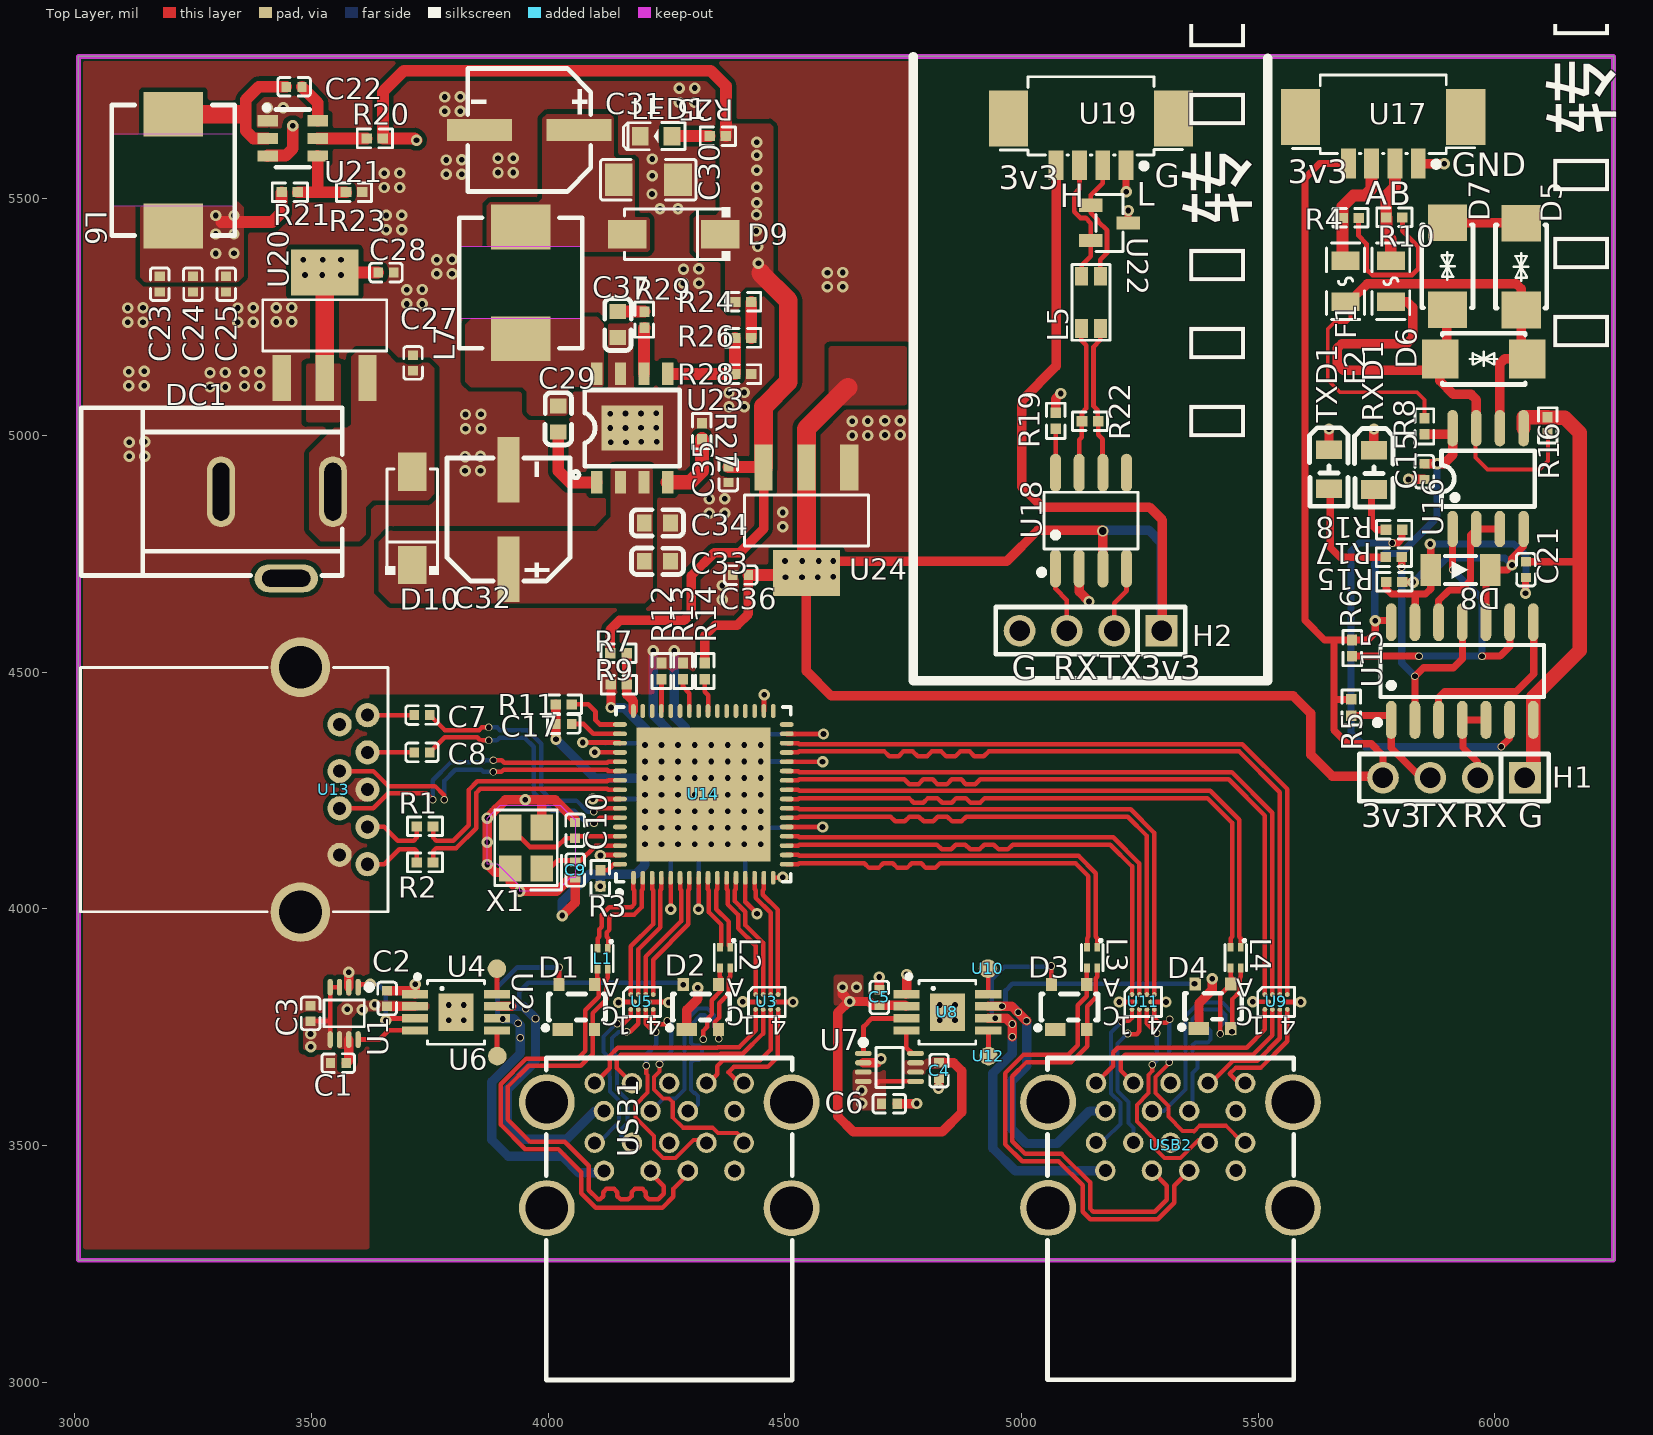
[diagram p0: Top Layer view]
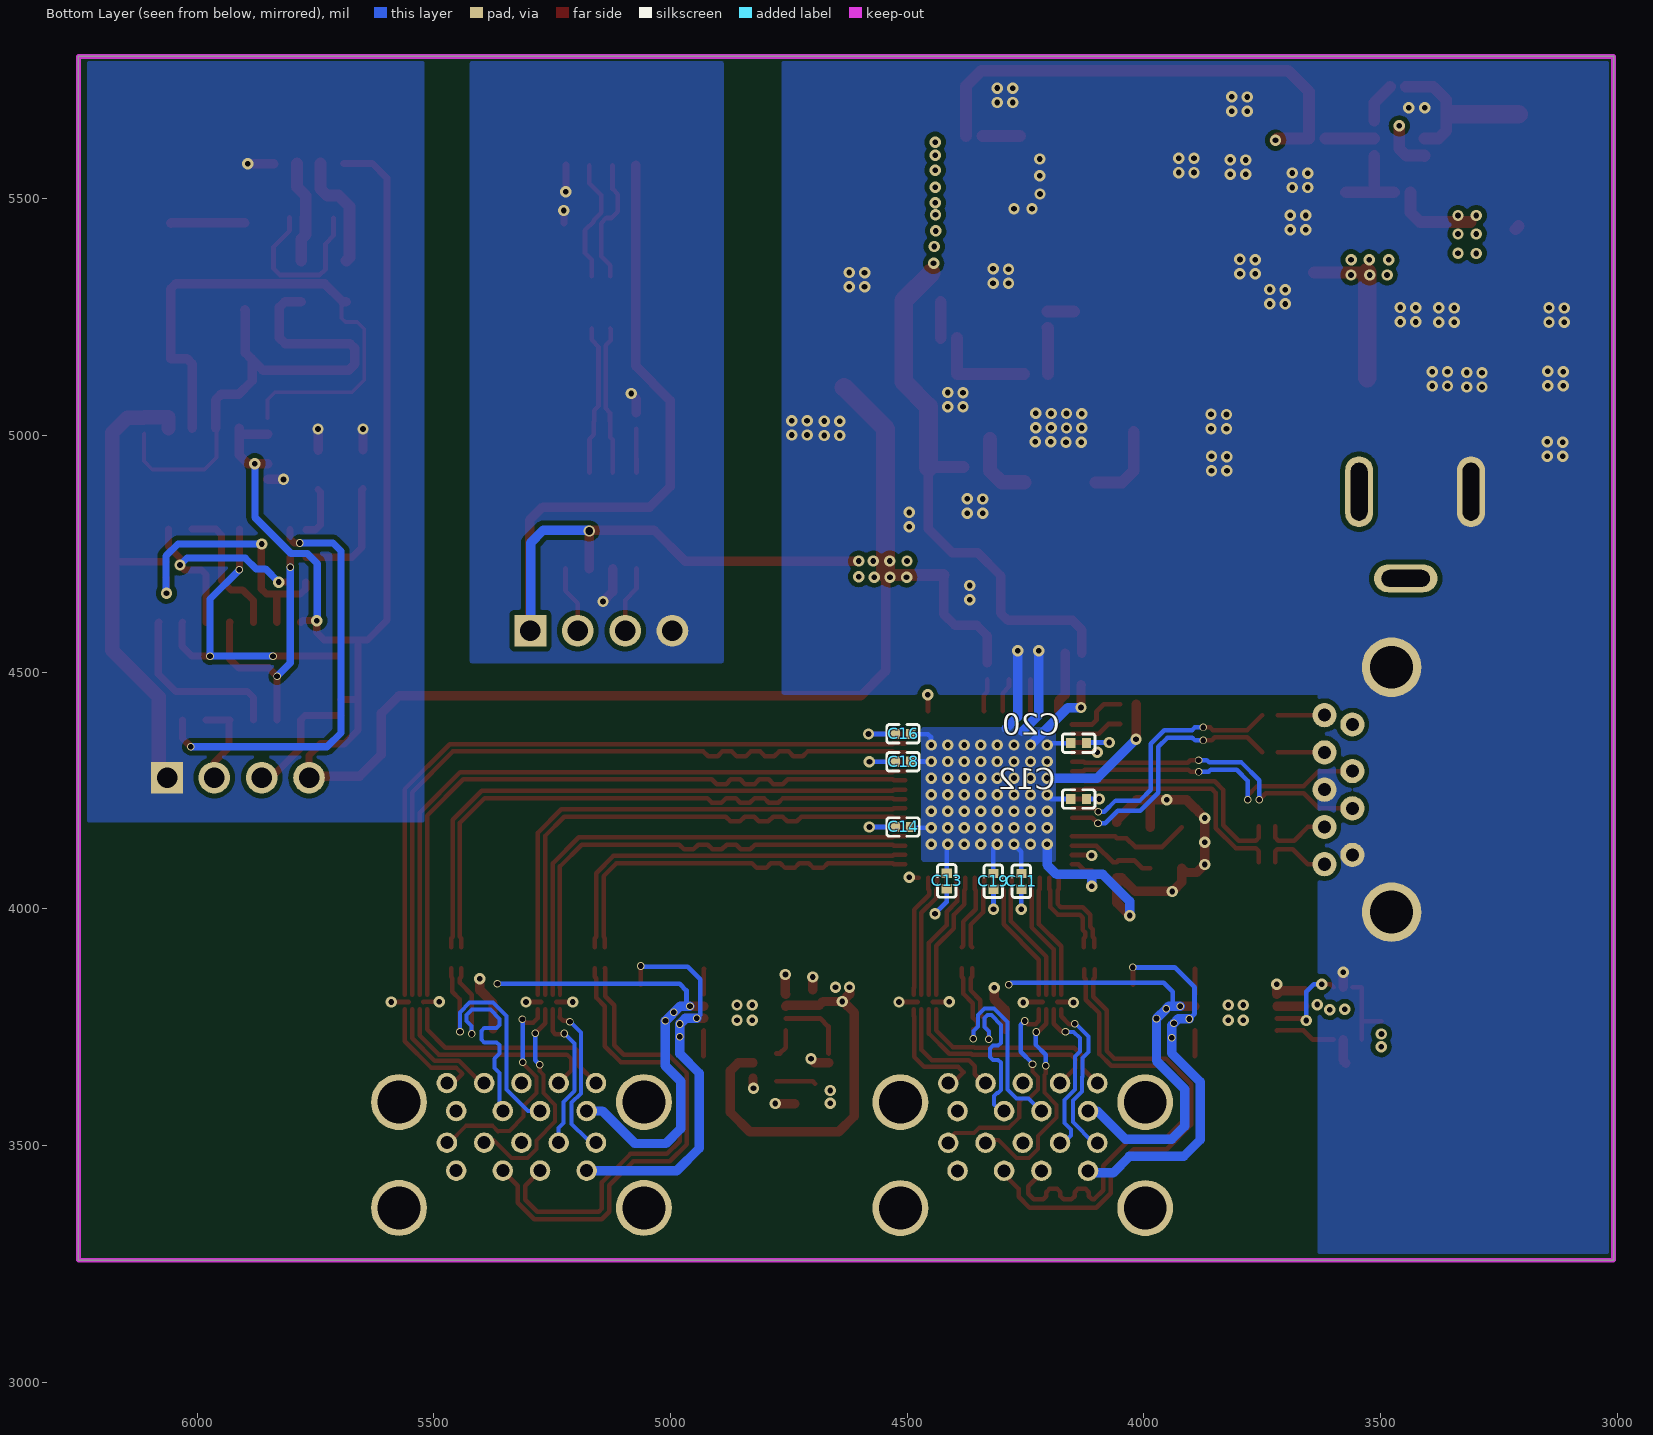
[diagram p1: Bottom Layer view, seen from below]
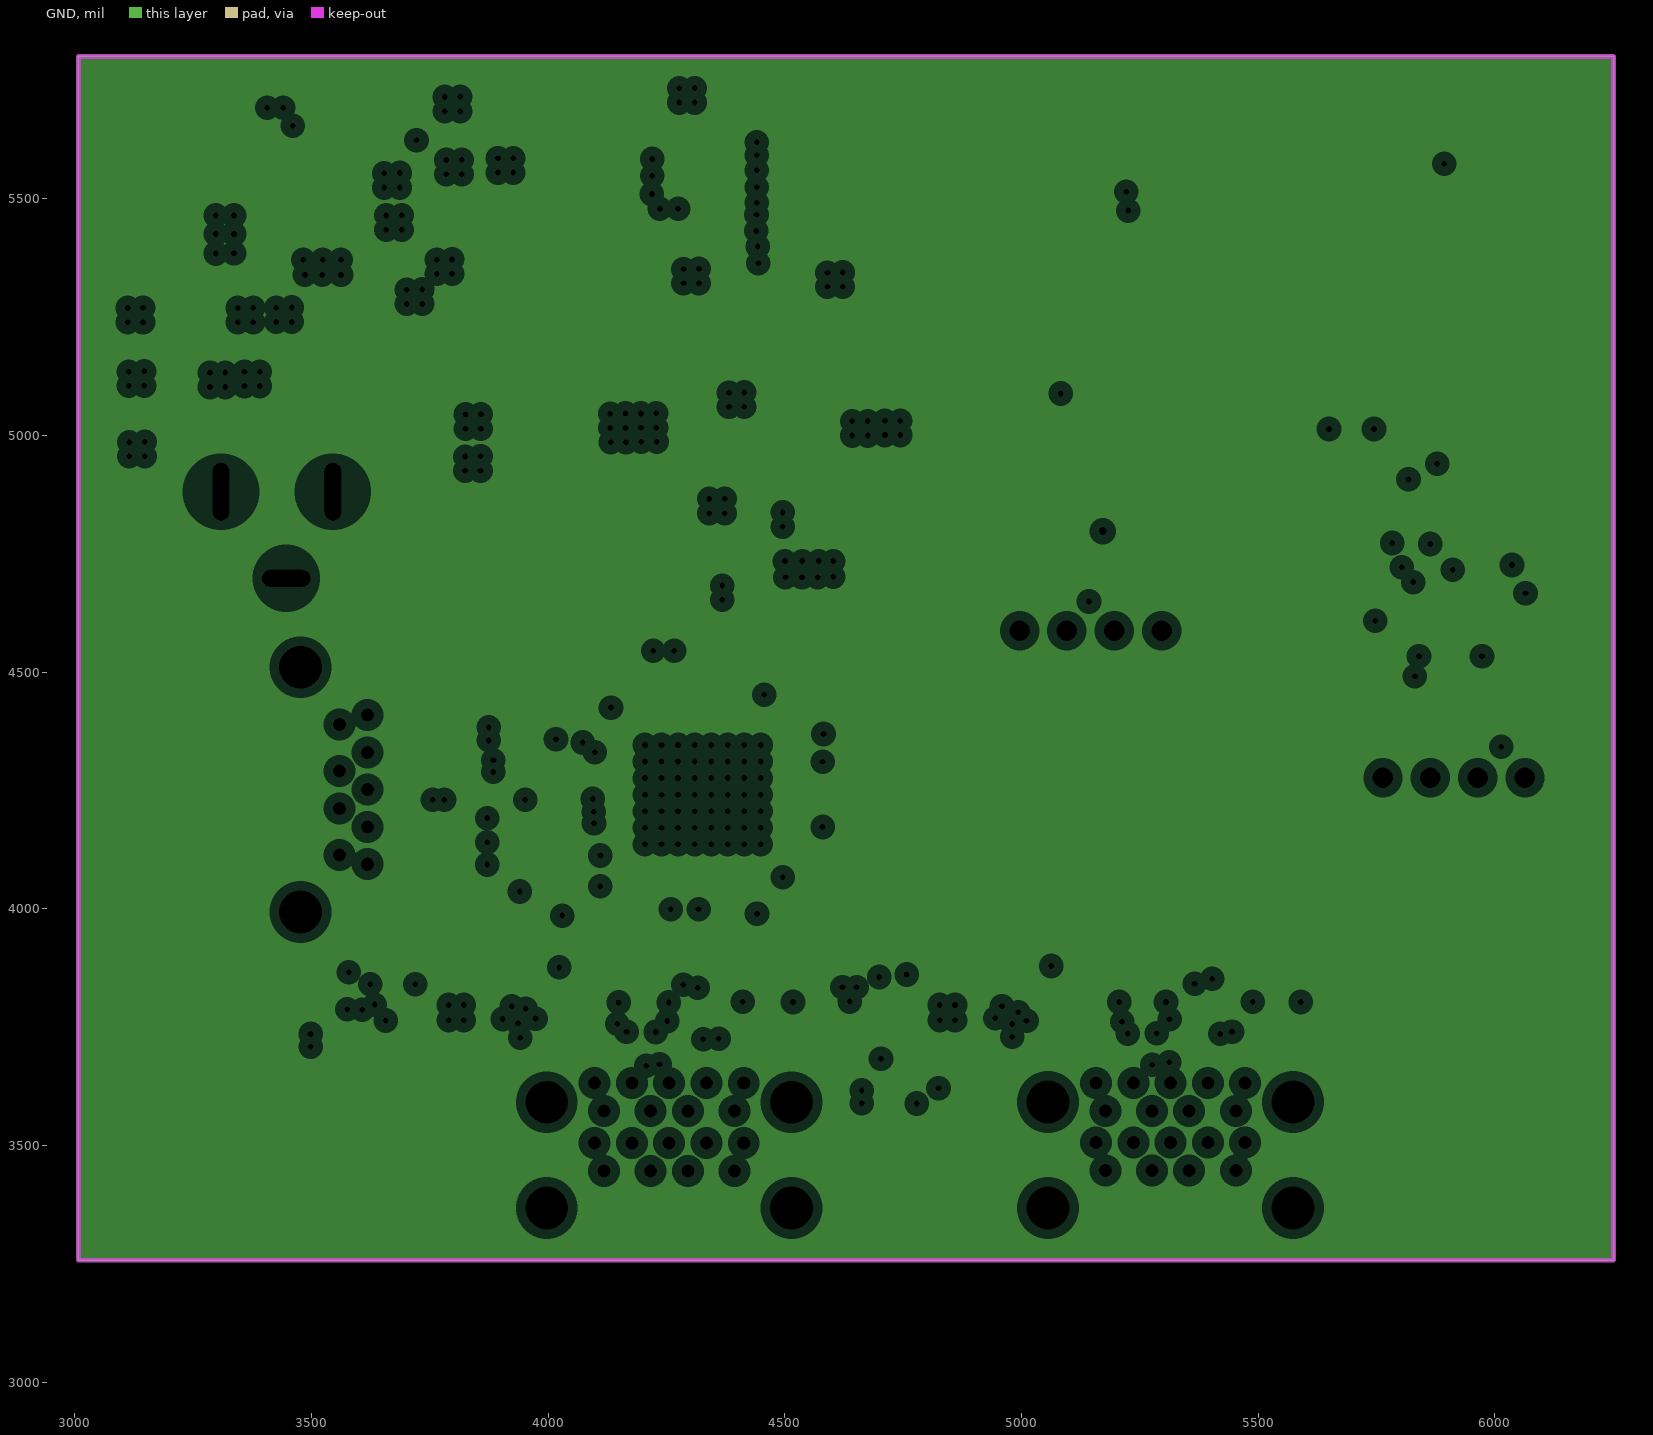
[diagram p2: GND, clearances drawn from the general rule]
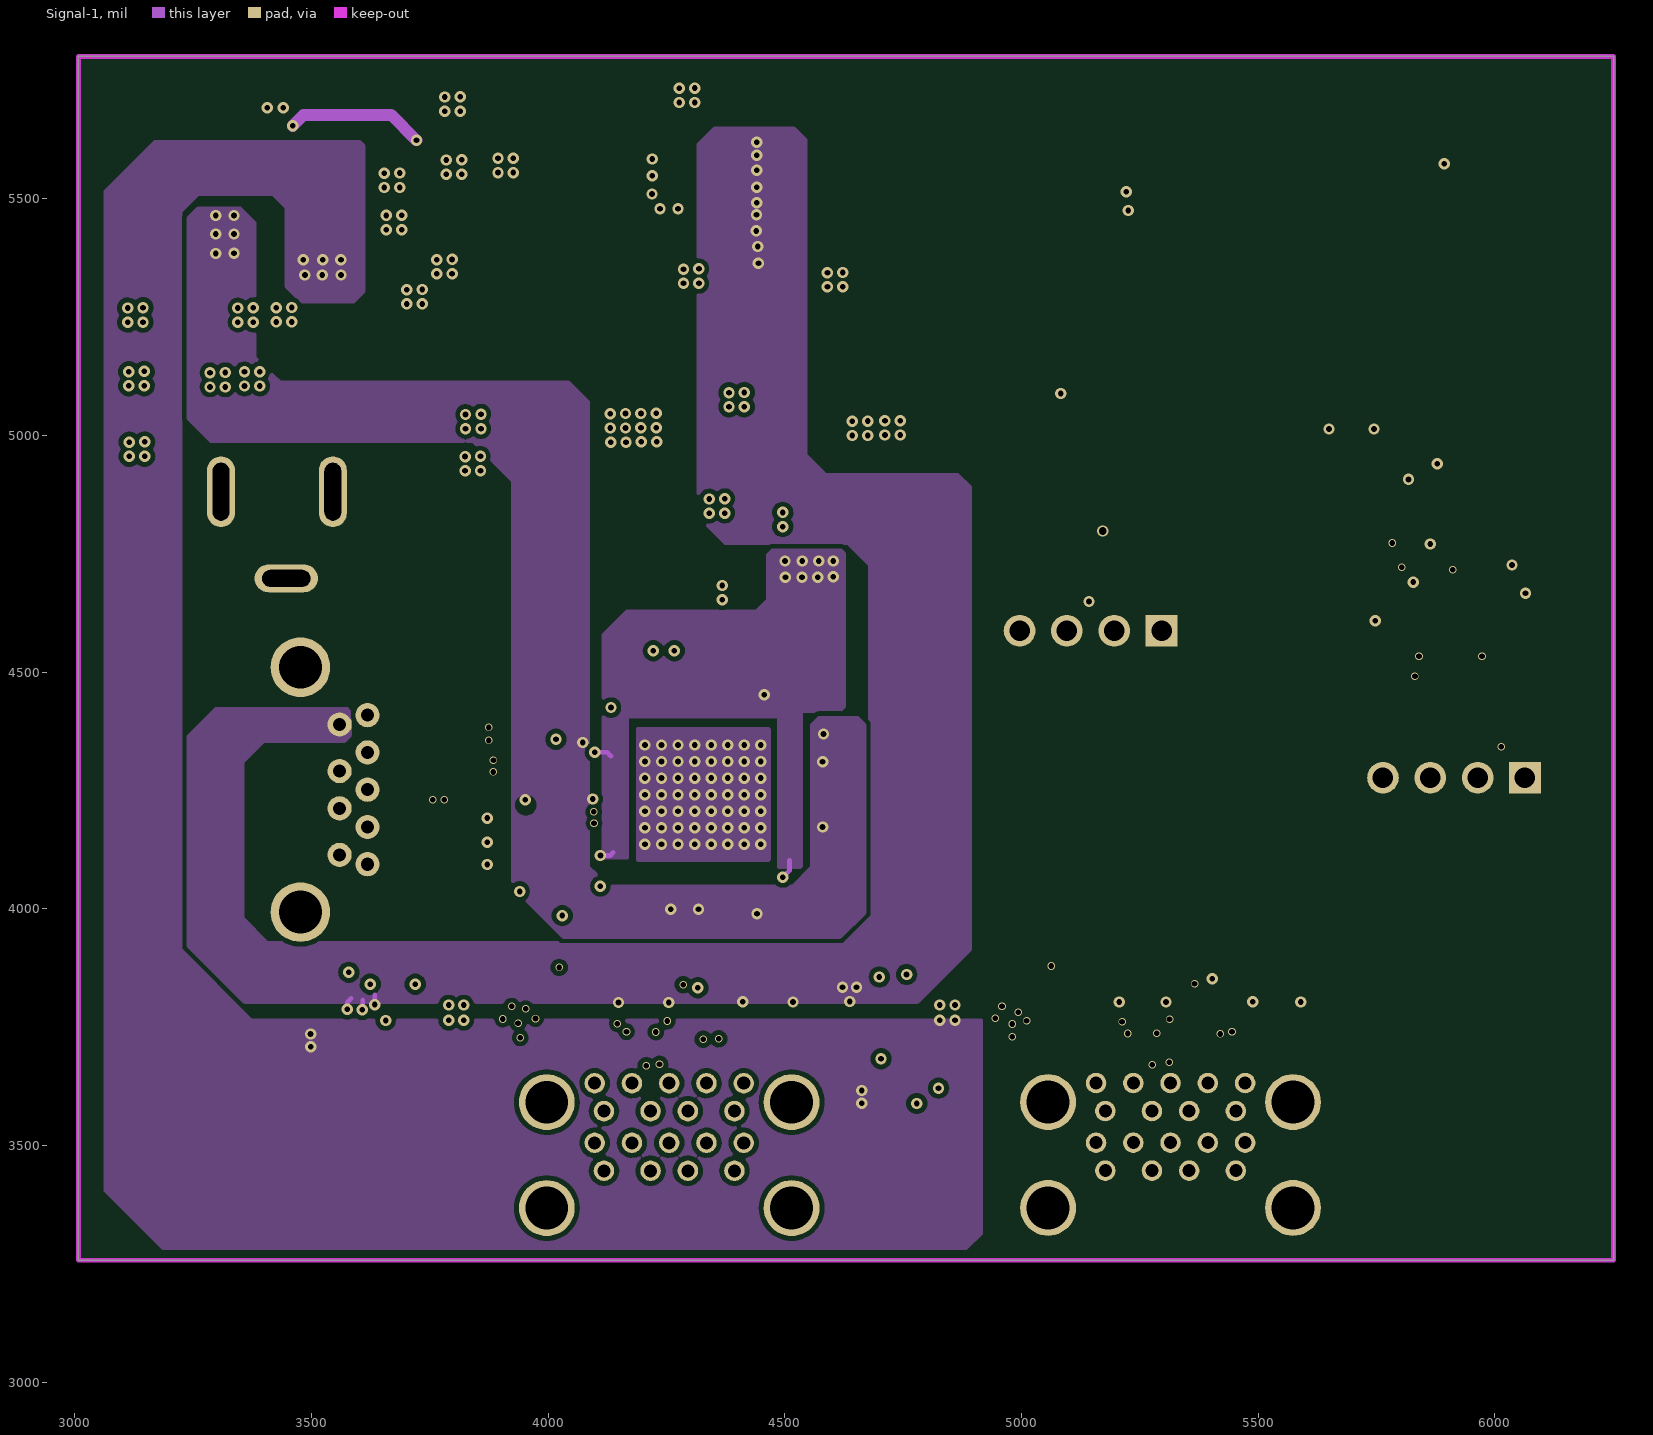
[diagram p3: Signal-1]
# Altium PCB MISC51972.pcbdoc (part 1 of 3)
Units mil, origin at the board's own origin, x right, y up, seen from the top; angles counter-clockwise.
Board outline 3243 x 2543 mil, 4 copper layers (Top Layer, GND, Signal-1, Bottom Layer), stack 62.447 mil thick; 117 components, 123 nets, 473 pads, 324 vias.

## Layer stack, top to bottom
Top Layer: signal copper 1.378
Dielectric1: surface 8.283, 7628 RC49% 8.6mil, Dk 0
GND: plane copper 0.598
Dielectric2: surface 41.929, 1.1mm H/HOZ Copper, Dk 0
Signal-1: signal copper 0.598
Dielectric3: surface 8.283, 7628 RC49% 8.6mil, Dk 0
Bottom Layer: signal copper 1.378

## Board outline
3007.5,5801 3007.5,3258 6250.5,3258 6250.5,5801

## Design rules (kind name [scope] priority, off if disabled: settings)
BoardOutlineClearance copperThickness2oz_1 [All] p2 off: genericclearance=7.99 ignorepadtopadclearanceinfootprint=FALSE except(0: Arc-SplitContinuation Track-SplitContinuation SMDPad-SplitContinuation THPad-SplitContinuation Via-SplitContinuation Fill-SplitContinuation Region-SplitContinuation Poly-SplitContinuation Text-SplitContinuation Hole-SplitContinuation; 5.98: Arc-CutoutEdge Track-CutoutEdge SMDPad-CutoutEdge THPad-CutoutEdge Via-CutoutEdge Text-CutoutEdge; 6.89: Hole-OutlineEdge Hole-CutoutEdge; 10: Poly-OutlineEdge Poly-CutoutEdge; 11.81: Arc-OutlineEdge Track-OutlineEdge SMDPad-OutlineEdge THPad-OutlineEdge Via-OutlineEdge Fill-OutlineEdge Region-OutlineEdge Text-OutlineEdge Fill-CutoutEdge Region-CutoutEdge)
BoardOutlineClearance Copper_copperRegion_1 [All] p4 off: genericclearance=3.5 ignorepadtopadclearanceinfootprint=FALSE except(0: Arc-SplitContinuation Track-SplitContinuation SMDPad-SplitContinuation THPad-SplitContinuation Via-SplitContinuation Fill-SplitContinuation Region-SplitContinuation Poly-SplitContinuation Text-SplitContinuation Hole-SplitContinuation; 0.98: Hole-OutlineEdge Hole-CutoutEdge; 5.98: SMDPad-CutoutEdge THPad-CutoutEdge Via-CutoutEdge Fill-CutoutEdge Region-CutoutEdge Text-CutoutEdge; 10: Poly-OutlineEdge Poly-CutoutEdge; 11.81: Arc-OutlineEdge Track-OutlineEdge SMDPad-OutlineEdge THPad-OutlineEdge Via-OutlineEdge Fill-OutlineEdge Region-OutlineEdge Text-OutlineEdge Arc-CutoutEdge Track-CutoutEdge)
BoardOutlineClearance Plane_innerPlane_1 [All] p6 off: genericclearance=3.5 ignorepadtopadclearanceinfootprint=FALSE except(0: Arc-SplitContinuation Track-SplitContinuation SMDPad-SplitContinuation THPad-SplitContinuation Via-SplitContinuation Fill-SplitContinuation Region-SplitContinuation Poly-SplitContinuation Text-SplitContinuation Hole-SplitContinuation; 0.98: Hole-OutlineEdge Hole-CutoutEdge; 5.98: SMDPad-CutoutEdge THPad-CutoutEdge Via-CutoutEdge Fill-CutoutEdge Region-CutoutEdge Text-CutoutEdge; 10: Poly-OutlineEdge Poly-CutoutEdge; 11.81: Arc-OutlineEdge Track-OutlineEdge SMDPad-OutlineEdge THPad-OutlineEdge Via-OutlineEdge Fill-OutlineEdge Region-OutlineEdge Text-OutlineEdge Arc-CutoutEdge Track-CutoutEdge)
BoardOutlineClearance copperThickness1oz_1 [All] p8: genericclearance=3.5 ignorepadtopadclearanceinfootprint=FALSE except(0: Arc-SplitContinuation Track-SplitContinuation SMDPad-SplitContinuation THPad-SplitContinuation Via-SplitContinuation Fill-SplitContinuation Region-SplitContinuation Poly-SplitContinuation Text-SplitContinuation Hole-SplitContinuation; 0.98: Hole-OutlineEdge Hole-CutoutEdge; 5.98: SMDPad-CutoutEdge THPad-CutoutEdge Via-CutoutEdge Fill-CutoutEdge Region-CutoutEdge Text-CutoutEdge; 10: Poly-OutlineEdge Poly-CutoutEdge; 11.81: Arc-OutlineEdge Track-OutlineEdge SMDPad-OutlineEdge THPad-OutlineEdge Via-OutlineEdge Fill-OutlineEdge Region-OutlineEdge Text-OutlineEdge Arc-CutoutEdge Track-CutoutEdge)
Clearance copperThickness2oz [All] p1 off: gap=7.99 ignorepadtopadclearanceinfootprint=FALSE except(5.98: SMDPad-Track SMDPad-SMDPad THPad-Track SMDPad-THPad THPad-THPad Track-Via SMDPad-Via THPad-Via Via-Via Fill-SMDPad Region-SMDPad Fill-THPad Region-THPad Fill-Via Region-Via Fill-Fill Fill-Region Region-Region Arc-Track Arc-SMDPad Arc-THPad Arc-Via Fill-Arc Region-Arc Arc-Arc Text-Track SMDPad-Text Text-THPad Text-Via Fill-Text Region-Text Arc-Text Text-Text; 6.89: Hole-Track Hole-SMDPad Hole-THPad Hole-Via Fill-Hole Region-Hole Hole-Arc Hole-Text; 10: Poly-Track Poly-SMDPad Poly-THPad Poly-Via Poly-Fill Poly-Region Poly-Poly Poly-Arc Poly-Text Poly-Hole; 11.81: Fill-Track Region-Track)
Clearance Copper_copperRegion [All] p3 off: gap=3.5 ignorepadtopadclearanceinfootprint=FALSE except(0.98: Hole-Track Hole-SMDPad Hole-THPad Hole-Via Fill-Hole Region-Hole Hole-Arc Hole-Text; 2.01: SMDPad-Via; 2.28: SMDPad-Track; 2.3: SMDPad-SMDPad SMDPad-THPad; 3.9: Track-Via; 5.98: THPad-Track THPad-THPad THPad-Via Via-Via Fill-Track Region-Track Fill-SMDPad Region-SMDPad Fill-THPad Region-THPad Fill-Via Region-Via Fill-Fill Fill-Region Region-Region Arc-Track Arc-SMDPad Arc-THPad Arc-Via Fill-Arc Region-Arc Arc-Arc Text-Track SMDPad-Text Text-THPad Text-Via Fill-Text Region-Text Arc-Text Text-Text; 10: Poly-Track Poly-SMDPad Poly-THPad Poly-Via Poly-Fill Poly-Region Poly-Poly Poly-Arc Poly-Text Poly-Hole)
Clearance Plane_innerPlane [All] p5 off: gap=3.5 ignorepadtopadclearanceinfootprint=FALSE except(0.98: Hole-Track Hole-SMDPad Hole-THPad Hole-Via Fill-Hole Region-Hole Hole-Arc Hole-Text; 2.01: SMDPad-Via; 2.28: SMDPad-Track; 2.3: SMDPad-SMDPad SMDPad-THPad; 3.9: Track-Via; 5.98: THPad-Track THPad-THPad THPad-Via Via-Via Fill-Track Region-Track Fill-SMDPad Region-SMDPad Fill-THPad Region-THPad Fill-Via Region-Via Fill-Fill Fill-Region Region-Region Arc-Track Arc-SMDPad Arc-THPad Arc-Via Fill-Arc Region-Arc Arc-Arc Text-Track SMDPad-Text Text-THPad Text-Via Fill-Text Region-Text Arc-Text Text-Text; 10: Poly-Track Poly-SMDPad Poly-THPad Poly-Via Poly-Fill Poly-Region Poly-Poly Poly-Arc Poly-Text Poly-Hole)
Clearance copperThickness1oz [All] p7: gap=3.5 ignorepadtopadclearanceinfootprint=FALSE except(0.98: Hole-Track Hole-SMDPad Hole-THPad Hole-Via Fill-Hole Region-Hole Hole-Arc Hole-Text; 2.01: SMDPad-Via; 2.28: SMDPad-Track; 2.3: SMDPad-SMDPad SMDPad-THPad; 3.9: Track-Via; 5.98: THPad-Track THPad-THPad THPad-Via Via-Via Fill-Track Region-Track Fill-SMDPad Region-SMDPad Fill-THPad Region-THPad Fill-Via Region-Via Fill-Fill Fill-Region Region-Region Arc-Track Arc-SMDPad Arc-THPad Arc-Via Fill-Arc Region-Arc Arc-Arc Text-Track SMDPad-Text Text-THPad Text-Via Fill-Text Region-Text Arc-Text Text-Text; 10: Poly-Track Poly-SMDPad Poly-THPad Poly-Via Poly-Fill Poly-Region Poly-Poly Poly-Arc Poly-Text Poly-Hole)
DiffPairsRouting CAN [All] p1 off: maxlimit=8 minlimit=6 mostfreqgap=8 toplayer_minwidth=5 toplayer_prefwidth=8 toplayer_maxwidth=100 toplayer_mingap=6 toplayer_prefgap=8 toplayer_maxgap=8 midlayer1_minwidth=5 midlayer1_prefwidth=8 midlayer1_maxwidth=100 midlayer1_mingap=6 midlayer1_prefgap=8 midlayer1_maxgap=8 bottomlayer_minwidth=5 bottomlayer_prefwidth=8 bottomlayer_maxwidth=100 bottomlayer_mingap=6 bottomlayer_prefgap=8 bottomlayer_maxgap=8 maxuncoupledlength=10
DiffPairsRouting usb2.0 [(InNet('USB30_T_DP1') OR InNet('$1N3807') OR InNet('$1N3806') OR InNet('$1N3821') OR InNet('$1N3814') OR InNet('$1N3813') OR InNet('$1N3822') OR InNet('$1N3831') OR InNet('$1N3827') OR InNet('USB30_T_DM1') OR InNet('USB30_T_DP2') OR InNet('USB30_T_DM2') OR InNet('USB30_T_DP3') OR InNet('USB30_T_DM3') OR InNet('USB30_T_DP4') OR InNet('USB30_T_DM4') OR InNet('USB30_USB_DM') OR InNet('USB30_USB_DP'))] p2: maxlimit=6 minlimit=5 mostfreqgap=6 toplayer_minwidth=8.4 toplayer_prefwidth=9.5 toplayer_maxwidth=9.5 toplayer_mingap=5 toplayer_prefgap=6 toplayer_maxgap=6 midlayer1_minwidth=8.4 midlayer1_prefwidth=9.5 midlayer1_maxwidth=9.5 midlayer1_mingap=5 midlayer1_prefgap=6 midlayer1_maxgap=6 bottomlayer_minwidth=8.4 bottomlayer_prefwidth=9.5 bottomlayer_maxwidth=9.5 bottomlayer_mingap=5 bottomlayer_prefgap=6 bottomlayer_maxgap=6 maxuncoupledlength=39.41
DiffPairsRouting usb3.0 [All] p3: maxlimit=6 minlimit=5 mostfreqgap=6 toplayer_minwidth=8.4 toplayer_prefwidth=9.5 toplayer_maxwidth=9.5 toplayer_mingap=5 toplayer_prefgap=6 toplayer_maxgap=6 midlayer1_minwidth=8.4 midlayer1_prefwidth=9.5 midlayer1_maxwidth=9.5 midlayer1_mingap=5 midlayer1_prefgap=6 midlayer1_maxgap=6 bottomlayer_minwidth=8.4 bottomlayer_prefwidth=9.5 bottomlayer_maxwidth=9.5 bottomlayer_mingap=5 bottomlayer_prefgap=6 bottomlayer_maxgap=6 maxuncoupledlength=25
HoleToHoleClearance otherClearance [All] p1: gap=11.81 allowstackedmicrovias=TRUE
Length netLength [All] p1: minlimit=0 maxlimit=0
PasteMaskExpansion pasteMaskExpansion [All] p1: expansion=0
PlaneConnect innerPlane [All] p1: planeconnectstyle=Direct reliefexpansion=20 reliefentries=4 reliefconductorwidth=10 reliefairgap=10
PolygonConnect copperRegion [All] p1: connectstyle=Direct reliefconductorwidth=10 reliefentries=4 polygonreliefangle="90 Angle" airgapwidth=10 via.connectstyle=Relief via.reliefconductorwidth=10 via.reliefentries=4 via.polygonreliefangle="90 Angle" via.airgapwidth=10
RoutingVias 信号 [All] p1 off: holewidth=8 width=14 viastyle="Through Hole" minholewidth=5 minwidth=10 maxholewidth=248.03 maxwidth=393.7
RoutingVias viaSize [All] p2: holewidth=12.01 width=24.02 viastyle="Through Hole" minholewidth=11.81 minwidth=15.75 maxholewidth=247.99 maxwidth=100
SolderMaskExpansion solderMaskExpansion [IsVia] p1: expansion=-1000 istentingtop=TRUE
SolderMaskExpansion solderMaskExpansion [All] p2: expansion=0.98 istentingtop=FALSE
Width copperThickness2oz_2 [All] p1 off: maxlimit=100 minlimit=8 preferedwidth=10
Width copperThickness1oz_2 [All] p2: maxlimit=100 minlimit=3.9 preferedwidth=20

## Components (designator, comment, footprint, x,y, rotation, side; value= is the part's Value field where it differs from the comment)
C1 "100nF" C0402 3556.5,3674.3 r0 top
C2 "100nF" C0402 3659.5,3811 r90 top
C3 "100nF" C0402 3497.8,3779.3 r90 top
C4 "100nF" C0402 4825.5,3658.5 r90 top
C5 "100nF" C0402 4699.5,3813 r90 top
C6 "100nF" C0402 4720.5,3588.5 r0 top
C7 "100nF" C0402 3733.25,4409.68 r0 top
C8 "100nF" C0402 3733.25,4330.78 r0 top
C9 "12pF" C0402 4057,4082.3 r90 top
C10 "12pF" C0402 4056.7,4166.1 r270 top
C11 "100nF" C0402 4258.6,4058.5 r270 bottom
C12 "100nF" C0402 4137.4,4232.3 r180 bottom
C13 "100nF" C0402 4416.1,4059.2 r270 bottom
C14 "100nF" C0402 4508.56,4173.2 r0 bottom
C15 "Cap" C0402 5851,4924 r270 top
C16 "100nF" C0402 4508.56,4370.1 r0 bottom
C17 "100nF" C0402 4032.8,4390.72 r180 top
C18 "100nF" C0402 4508.56,4311 r0 bottom
C19 "100nF" C0402 4317.8,4058.5 r270 bottom
C20 "100nF" C0402 4137.4,4350.3 r180 bottom
C21 "Cap" C0402 6065.5,4717 r270 top
C22 "100nF" C0402 3463,5737 r0 top
C23 "22uF" C0402 3179.2,5319.9 r90 top
C24 "22uF" C0402 3249.35,5319.9 r90 top
C25 "100nF" C0402 3319.5,5319.9 r90 top
C27 "10uF" C0402 3714.3,5153.56 r270 top
C28 "22uF" C0402 3657,5344.5 r180 top
C29 "100nF" C0603 4021.1,5035.16 r270 top
C30 "47uF" C1206 4211.5,5540.5 r180 top
C31 "220uF" CAP-SMD_BD6.3-L6.5-W6.5-LS7.2-FD 3959.9,5645.7 r180 top
C32 "100uF" CAP-SMD_BD6.3-L6.5-W6.5-LS7.0-FD 3916,4822.7 r90 top
C33 "4.7uF" C0603 4230.4,4734.6 r180 top
C34 "100nF" C0603 4230.4,4815.7 r180 top
C35 "10uF" C0402 4380.5,4917.5 r90 top
C36 "22uF" C0402 4406.3,4705.5 r0 top
C37 "4.7nF" C0603 4147,5234.5 r270 top
D1 "CD143A-SR05" SOT-143_L2.9-W1.3-P1.92-LS2.3-BL 4060,3792.8 r0 top
D2 "CD143A-SR05" SOT-143_L2.9-W1.3-P1.92-LS2.3-BL 4322.4,3792.8 r0 top
D3 "CD143A-SR05" SOT-143_L2.9-W1.3-P1.92-LS2.3-BL 5100.3,3792.8 r0 top
D4 "CD143A-SR05" SOT-143_L2.9-W1.3-P1.92-LS2.3-BL 5404.3,3794.3 r0 top
D5 "SMAJ6.5CA" SMA-L4.3-W2.6-LS5.3-BI 6055.45,5357.16 r90 top
D6 "SMAJ6.5CA" SMA-L4.3-W2.6-LS5.3-BI 5976.5,5162 r0 top
D7 "SMAJ6.5CA" SMA-L4.3-W2.6-LS5.3-BI 5899.45,5357.66 r270 top
D8 "LL4148" LL-34_L3.5-W1.5-RD 5927.45,4716.16 r180 top
D9 "SS54" SMA_L4.4-W2.8-LS5.4-R-RD 4265.2,5425.6 r180 top
D10 "SS54" SMA_L4.4-W2.8-LS5.4-R-RD 3712.5,4825.3 r90 top
DC1 "DC-005-A200" DC-IN-TH_DC-005-A200 3426.8,4790 r0 top
F1 "SMD0805-010-33" F0805 5684.45,5326.16 r90 top
F2 "SMD0805-010-33" F0805 5779.95,5326.16 r90 top
H1 "PZ254V-11-04P" HDR-TH_4P-P2.54-V-M 5913.5,4277.5 r180 top
H2 "PZ254V-11-04P" HDR-TH_4P-P2.54-V-M 5145.64,4587.86 r180 top
L1 "DLM11SN900HY2L" FILTER-SMD_4P-L1.3-W1.0-TL_DLP11SN201HL2L 4114.6,3895.1 r270 top
L2 "DLM11SN900HY2L" FILTER-SMD_4P-L1.3-W1.0-TL_DLP11SN201HL2L 4373.5,3897.1 r270 top
L3 "DLM11SN900HY2L" FILTER-SMD_4P-L1.3-W1.0-TL_DLP11SN201HL2L 5149,3897.1 r270 top
L4 "DLM11SN900HY2L" FILTER-SMD_4P-L1.3-W1.0-TL_DLP11SN201HL2L 5452.4,3897.1 r270 top
L5 "744232102" IND-SMD_4P-L3.2-W1.6 5146.64,5281.36 r90 top
L6 "3.3uH" IND-SMD_L7.0-W6.6#1 3207.9,5560.8 r90 top
L7 "4.7uH" IND-SMD_L7.0-W6.6#2 3941.9,5322.5 r90 top
LED1 "15-21VGC/TR8" LED0603_GREEN 4228,5632.7 r180 top
R1 "0R" R0402 3739.45,4174.48 r0 top
R2 "0R" R0402 3739.45,4098.28 r0 top
R3 "9.53K" R0402 4110,4065 r270 top
R4 "Res1" R0402 5694.95,5460.16 r0 top
R5 "Res1" R0402 5696.45,4425.66 r90 top
R6 "Res1" R0402 5698.45,4551.16 r90 top
R7 "90.9K" R0402 4148.29,4540.28 r180 top
R8 "Res1" R0402 5851,5019.5 r270 top
R9 "10K" R0402 4149.16,4473.9 r180 top
R10 "Res1" R0402 5787.45,5461.16 r0 top
R11 "4.7K" R0402 4032.8,4432.4 r180 top
R12 "4.7K" R0402 4239.1,4502.6 r90 top
R13 "4.7K" R0402 4284.8,4502.6 r90 top
R14 "4.7K" R0402 4330.6,4502.6 r90 top
R15 "Res1" R0402 5787.49,4691.16 r180 top
R16 "Res1" R0402 6111.45,5021.62 r270 top
R17 "Res1" R0402 5786.45,4743.16 r180 top
R18 "Res1" R0402 5786.91,4801.16 r0 top
R19 "10K" R0402 5072.14,5031.4 r90 top
R20 "10kΩ" R0402 3633.6,5627.9 r0 top
R21 "4.3kΩ" R0402 3453.9,5514.3 r180 top
R22 "120R 1%" R0402 5144.64,5030.36 r180 top
R23 "10kΩ" R0402 3589.7,5514.3 r0 top
R24 "51kΩ" R0402 4411.7,5282.6 r0 top
R25 "4.7kΩ" R0402 4358.2,5632.7 r180 top
R26 "1.5kΩ" R0402 4411.7,5206.35 r180 top
R27 "200kΩ" R0402 4324.5,5009.36 r270 top
R28 "10kΩ" R0402 4411.7,5130.1 r0 top
R29 "20kΩ" R0402 4203,5245 r90 top
RXD1 "GL0805UR01" LED0805-R-RD_RED 5744.45,4927.66 r270 top
TXD1 "GL0805UR01" LED0805-R-RD_RED 5649.45,4929.16 r270 top
U1 "TXS0102DCUT" VSSOP-8_L2.3-W2.0-P0.50-LS3.1-BR 3568.8,3779.4 r90 top
U2 "TPS2060CDGNR" HVSSOP-8_L3.0-W3.0-P0.65-LS4.9-BL-EP-1 3805.1,3781.6 r270 top
U3 "" PCMF2USB3S 4461.75,3803.51 r90 top
U4 "" tp点 3896.5,3873.8 r0 top
U5 "" PCMF2USB3S 4198,3803.51 r90 top
U6 "" tp点 3897.3,3689.1 r0 top
U7 "TXS0102DCUT" VSSOP-8_L2.3-W2.0-P0.50-LS3.1-BR 4720.77,3665.28 r180 top
U8 "TPS2060CDGNR" HVSSOP-8_L3.0-W3.0-P0.65-LS4.9-BL-EP-1 4843,3781.6 r270 top
U9 "" PCMF2USB3S 5537.7,3803.51 r90 top
U10 "" tp点 4924,3873.8 r180 top
U11 "" PCMF2USB3S 5256.85,3803.51 r90 top
U12 "" tp点 4925,3689.1 r180 top
U13 "HC-USB3.0-L168-WP" USB-TH_USB3.0-A 3547.25,4251.98 r270 top
U14 "TUSB8041IRGCR" QFN-64_L9.0-W9.0-P0.50-BL-EP7.2 4327.59,4242.1 r0 top
U15 "74HC04D,653" SOIC-14_L8.7-W3.9-P1.27-LS6.0-BL 5930.95,4502.66 r0 top
U16 "SP3485EN-L/TR" SOIC-8_L5.0-W4.0-P1.27-LS6.0-BL 5985.45,4909.16 r0 top
U17 "ZX-MX1.25-4PWT" CONN-SMD_4P-P1.25-MX1.25-4P-WT 5763.95,5623.86 r180 top
U18 "SN65HVD230DR" SOIC-8_L4.9-W3.9-P1.27-LS6.0-BL 5146.64,4820.36 r0 top
U19 "ZX-MX1.25-4PWT" CONN-SMD_4P-P1.25-MX1.25-4P-WT 5146.64,5620.36 r180 top
U20 "AMS1117-1.8" SOT-223-4_L6.5-W3.5-P2.30-LS7.0-BR 3527.7,5233 r270 top
U21 "TPS563201DDCR" SOT-23-6_L2.9-W1.6-P0.95-LS2.8-BR 3460,5628 r180 top
U22 "SM24CANA-02HTG" SOT-23-3_L2.9-W1.3-P1.90-LS2.4-BR 5185.64,5449.36 r180 top
U23 "SCT2450STER" ESOP-8_L4.9-W3.9-P1.27-LS6.0-BL-EP 4177.3,5015.9 r0 top
U24 "AMS1117-3.3" SOT-223-4_L6.5-W3.5-P2.30-LS7.0-BR 4545.4,4820.9 r90 top
USB1 "HC-USB3.0-L175-2X1-P" USB-A-TH_H181-AF2R06-12ALCR 4255.5,3500 r0 top
USB2 "HC-USB3.0-L175-2X1-P" USB-A-TH_H181-AF2R06-12ALCR 5314.68,3500.3 r0 top
X1 "24MHz" CRYSTAL-SMD_4P-L3.2-W2.5-BL 3953,4129.2 r90 top

## Footprints (in the part's own frame and the unit in brackets; to place one, negate y for a bottom-side part, rotate by r counter-clockwise, add the part's x,y. Pads: shape width x height; smd on the part's side, far side on the other; paste and mask are expansions set on the pad)
C0402 [mm]
  rect 0.5x0.54 smd: 1(-0.42,0) 2(0.42,0)
  silkscreen extent -0.87,-0.5 0.87,0.5
C0603 [mm]
  rect 0.8x0.9 smd: 1(-0.7,0) 2(0.7,0)
  silkscreen extent -1.41,-0.71 1.39,0.72
C1206 [mm]
  rect 1.485x1.728 smd paste-100 mask+0.051: 1(-1.593,0) 2(1.593,0)
  silkscreen extent -2.56,-1.09 2.56,1.09
CAP-SMD_BD6.3-L6.5-W6.5-LS7.0-FD [mm]
  rect 3.5x1.2 smd paste+0 mask+0.051: 1(-2.67,0) 2(2.67,0)
  silkscreen extent -3.3,-3.3 3.3,3.3
CAP-SMD_BD6.3-L6.5-W6.5-LS7.2-FD [mm]
  rect 3.5x1.2 smd paste+0 mask+0.051: 1(-2.67,0) 2(2.67,0)
  silkscreen extent -3.3,-3.3 3.3,3.3
CONN-SMD_4P-P1.25-MX1.25-4P-WT [mm]
  rect 0.8x1.6 smd paste+0 mask+0.05: 1(-1.88,1.25) 2(-0.63,1.25) 3(0.62,1.25) 4(1.87,1.25)
  rect 2.1x3 smd paste+0 mask+0.05: 5(4.43,-1.25) 6(-4.43,-1.25)
  silkscreen extent -4.9,-3.5 4.87,1.43
CRYSTAL-SMD_4P-L3.2-W2.5-BL [mm]
  rect 1.4x1.2 smd: 1(-1.1,-0.85) 2(1.1,-0.85) 3(1.1,0.85) 4(-1.1,0.85)
  silkscreen extent -2.26,-1.91 2.03,1.68
DC-IN-TH_DC-005-A200 [mm]
  oval 1.5x3.8 hole 0.9 slot 3.1 at 90 deg copper offset -0.001,0: 1(3.001,2.325)
  oval 1.5x3.8 hole 0.9 slot 3.1 at 90 deg copper offset 0,0: 2(-3,2.325)
  oval 3.4x1.5 hole 0.9 slot 2.6 at 0 deg copper offset 0,-0.001: 3(0.5,-2.325)
  silkscreen extent -10.5,-2.17 3.5,6.83
ESOP-8_L4.9-W3.9-P1.27-LS6.0-BL-EP [mm]
  rect 0.6x1.2 smd paste+0 mask+0.051: 1(-1.905,-2.908) 2(-0.635,-2.908) 3(0.635,-2.908) 4(1.905,-2.908) 5(1.905,2.908) 6(0.635,2.908) 7(-0.635,2.908) 8(-1.905,2.908)
  rect 3.3x2.4 smd paste+0 mask+0.051: 9(0,0)
  silkscreen extent -3.2,-2.67 2.55,2.05
F0805 [mm]
  rect 1x1.5 smd paste-100 mask+0.051: 1(-1.1,0) 2(1.1,0)
  silkscreen extent -2.06,-1.02 2.06,1.02
FILTER-SMD_4P-L1.3-W1.0-TL_DLP11SN201HL2L [mm]
  rect 0.465x0.308 smd: 1(-0.558,0.275) 2(0.558,0.275) 3(0.558,-0.275) 4(-0.558,-0.275)
  silkscreen extent -0.99,-0.58 0.7,0.58
HDR-TH_4P-P2.54-V-M [mm]
  rect 1.7x1.7 hole 1.1: 1(-3.81,0)
  round 1.7 hole 1.1: 2(-1.27,0) 3(1.27,0) 4(3.81,0)
  silkscreen extent -5.08,-1.27 5.08,1.27
HVSSOP-8_L3.0-W3.0-P0.65-LS4.9-BL-EP-1 [mm]
  rect 0.45x1.4 smd paste+0 mask+0.05: 1(-0.975,-2.2) 2(-0.325,-2.2) 3(0.325,-2.2) 4(0.975,-2.2) 5(0.975,2.2) 6(0.325,2.2) 7(-0.325,2.2) 8(-0.975,2.2)
  rect 2x1.88 smd paste+0 mask+0.05: 9(0,0)
  silkscreen extent -2.03,-2.18 1.71,1.52
IND-SMD_4P-L3.2-W1.6 [mm]
  rect 1x0.7 smd: 1(-1.4,-0.5) 2(1.4,-0.5) 3(1.4,0.5) 4(-1.4,0.5)
  silkscreen extent -2.03,-1.02 2.03,1.02
IND-SMD_L7.0-W6.6#1 [mm]
  rect 2.4x3.2 smd: 1(-3,0) 2(3,0)
  silkscreen extent -3.5,-3.3 3.5,3.3
IND-SMD_L7.0-W6.6#2 [mm]
  rect 2.4x3.2 smd paste+0 mask+0.051: 1(-3,0) 2(3,0)
  silkscreen extent -3.5,-3.3 3.5,3.3
LED0603_GREEN [mm]
  rect 0.9x1 smd: 1(-0.85,0) 2(0.85,0)
  silkscreen extent -1.54,-0.73 1.75,0.73
LED0805-R-RD_RED [mm]
  rect 1x1.4 smd: 1(1.05,0) 2(-1.05,0)
  silkscreen extent -2.22,-1.04 1.99,1.01
LL-34_L3.5-W1.5-RD [mm]
  rect 1.1x1.7 smd: 1(-1.6,0) 2(1.6,0)
  silkscreen extent -0.85,-0.75 0.85,0.75
PCMF2USB3S [mil]
  round 10 smd: A1(15.75,23.62) A2(15.75,7.87) A3(15.75,-7.87) A4(15.75,-23.62) B1(0,15.75) B2(0,-15.75) C1(-15.75,23.62) C2(-15.75,7.87) C3(-15.75,-7.87) C4(-15.75,-23.62)
  silkscreen extent -31,-39 31,39
QFN-64_L9.0-W9.0-P0.50-BL-EP7.2 [mm]
  oval 0.25x0.75 smd paste-100 mask+0.051: 1(-3.75,-4.475) 2(-3.25,-4.475) 3(-2.75,-4.475) 4(-2.25,-4.475) 5(-1.75,-4.475) 6(-1.25,-4.475) 7(-0.75,-4.475) 8(-0.25,-4.475) 9(0.25,-4.475) 10(0.75,-4.475) 11(1.25,-4.475) 12(1.75,-4.475) 13(2.25,-4.475) 14(2.75,-4.475) 15(3.25,-4.475) 16(3.75,-4.475) 33(3.75,4.475) 34(3.25,4.475) 35(2.75,4.475) 36(2.25,4.475) 37(1.75,4.475) 38(1.25,4.475) 39(0.75,4.475) 40(0.25,4.475) 41(-0.25,4.475) 42(-0.75,4.475) 43(-1.25,4.475) 44(-1.75,4.475) 45(-2.25,4.475) 46(-2.75,4.475) 47(-3.25,4.475) 48(-3.75,4.475)
  oval 0.75x0.25 smd paste-100 mask+0.051: 17(4.475,-3.75) 18(4.475,-3.25) 19(4.475,-2.75) 20(4.475,-2.25) 21(4.475,-1.75) 22(4.475,-1.25) 23(4.475,-0.75) 24(4.475,-0.25) 25(4.475,0.25) 26(4.475,0.75) 27(4.475,1.25) 28(4.475,1.75) 29(4.475,2.25) 30(4.475,2.75) 31(4.475,3.25) 32(4.475,3.75) 49(-4.475,3.75) 50(-4.475,3.25) 51(-4.475,2.75) 52(-4.475,2.25) 53(-4.475,1.75) 54(-4.475,1.25) 55(-4.475,0.75) 56(-4.475,0.25) 57(-4.475,-0.25) 58(-4.475,-0.75) 59(-4.475,-1.25) 60(-4.475,-1.75) 61(-4.475,-2.25) 62(-4.475,-2.75) 63(-4.475,-3.25) 64(-4.475,-3.75)
  rect 7.2x7.2 smd paste-100 mask+0.051: 65(0,0)
  silkscreen extent -4.69,-5.4 4.69,4.69
R0402 [mm]
  rect 0.566x0.54 smd paste-100 mask+0.051: 1(-0.433,0) 2(0.433,0)
  silkscreen extent -0.94,-0.5 0.94,0.5
SMA-L4.3-W2.6-LS5.3-BI [mm]
  rect 1.96x2.1 smd: 1(-2.33,0) 2(2.33,0)
  silkscreen extent -2.23,-1.38 2.23,1.38
SMA_L4.4-W2.8-LS5.4-R-RD [mil]
  rect 81.2x60.59 smd paste+0 mask+2: 1(98.57,0) 2(-98.57,0)
  silkscreen extent -119,-56 104,56
SOIC-8_L4.9-W3.9-P1.27-LS6.0-BL [mm]
  oval 0.588x2.045 smd: 1(-1.905,-2.57) 2(-0.635,-2.57) 3(0.635,-2.57) 4(1.905,-2.57) 5(1.905,2.57) 6(0.635,2.57) 7(-0.635,2.57) 8(-1.905,2.57)
  silkscreen extent -2.8,-2.92 2.53,1.52
SOIC-8_L5.0-W4.0-P1.27-LS6.0-BL [mil]
  oval 22.38x76.78 smd: 1(-75,-106.5) 2(-25,-106.5) 3(25,-106.5) 4(75,-106.5) 5(75,106.5) 6(25,106.5) 7(-25,106.5) 8(-75,106.5)
  silkscreen extent -98,-59 98,59
SOIC-14_L8.7-W3.9-P1.27-LS6.0-BL [mil]
  oval 22.6x80.24 smd: 1(-150,-103.11) 2(-100,-103.11) 3(-50,-103.11) 4(0,-103.11) 5(50,-103.11) 6(100,-103.11) 7(150,-103.11) 8(150,103.11) 9(100,103.11) 10(50,103.11) 11(0,103.11) 12(-50,103.11) 13(-100,103.11) 14(-150,103.11)
  silkscreen extent -185,-115 172,55
SOT-23-3_L2.9-W1.3-P1.90-LS2.4-BR [mm]
  rect 1.25x0.7 smd: 1(1,-0.95) 2(1,0.95) 3(-1,0)
  silkscreen extent -0.73,-1.53 0.73,1.53
SOT-23-6_L2.9-W1.6-P0.95-LS2.8-BR [mm]
  rect 1.1x0.6 smd paste+0 mask+0.051: 1(1.35,-0.95) 2(1.35,0) 3(1.35,0.95) 4(-1.35,0.95) 5(-1.35,0) 6(-1.35,-0.95)
  silkscreen extent -0.9,-1.78 1.52,1.55
SOT-143_L2.9-W1.3-P1.92-LS2.3-BL [mm]
  rect 1.1x0.7 smd paste+0 mask+0.05: 1(-0.75,-1.2)
  rect 0.6x0.7 smd paste+0 mask+0.05: 2(0.95,-1.2) 3(0.95,1.2) 4(-0.95,1.2)
  silkscreen extent -1.8,-1.24 1.55,0.7
SOT-223-4_L6.5-W3.5-P2.30-LS7.0-BR [mm]
  rect 2.47x0.98 smd: 1(2.835,-2.3) 2(2.835,0) 3(2.835,2.3)
  rect 2.47x3.6 smd: 4(-2.835,0)
  silkscreen extent -1.37,-3.33 1.37,3.33
tp点 [mm]
  round 1 smd: 1(-0.127,0)
USB-A-TH_H181-AF2R06-12ALCR [mm]
  round 1.1 hole 0.7 paste+0 mask+0.05: 1(-3.5,-1.35) 2(-1,-1.35) 3(1,-1.35) 4(3.5,-1.35) 5(4,0.15) 6(2,0.15) 7(0,0.15) 8(-2,0.15) 9(-4,0.15) 10(-3.5,1.85) 11(-1,1.85) 12(1,1.85) 13(3.5,1.85) 14(4,3.35) 15(2,3.35) 16(0,3.35) 17(-2,3.35) 18(-4,3.35)
  round 3 hole 2.3 copper offset 0,0: 19(-6.57,2.33) 20(6.57,2.33)
  round 3 hole 2.3: 19(-6.57,-3.35) 20(6.57,-3.35)
  silkscreen extent -6.6,-12.57 6.6,4.7
USB-TH_USB3.0-A [mm]
  round 1.3 hole 0.7 paste+0 mask+0.05: 1(-3.5,0.3) 2(-1,0.3) 3(1,0.3) 4(3.5,0.3) 5(4,1.8) 6(2,1.8) 7(0,1.8) 8(-2,1.8) 9(-4,1.8)
  round 3.2 hole 2.3 paste+0 mask+0.05: 10(-6.57,-1.8) 10(6.57,-1.8)
  silkscreen extent -6.55,-13.6 6.55,2.9
VSSOP-8_L2.3-W2.0-P0.50-LS3.1-BR [mm]
  oval 0.905x0.28 smd: 1(1.403,-0.75) 2(1.403,-0.25) 3(1.403,0.25) 4(1.403,0.75) 5(-1.403,0.75) 6(-1.403,0.25) 7(-1.403,-0.25) 8(-1.403,-0.75)
  silkscreen extent -0.72,-1.49 1.55,1.08

## Via types
v1: diameter 24.02, hole 12, Top Layer to Bottom Layer, 276 vias
v2: diameter 16, hole 12, Top Layer to Bottom Layer, 47 vias
v3: diameter 24, hole 16, Top Layer to Bottom Layer, 1 vias

## Nets (pads, with @x,y where several pads share a name; then routed paths per layer and width w, separated by ;. In a path a pad name is that pad's centre, name@x,y a point inside that pad or via, vN(x,y) a via of type N, cw(c..) or ccw(c..) an arc to the next point about the centre after c; other vN are vias at no path point)
1.1V: C11.2 C12.2 C13.2 C14.2 C16.2 C18.2 C19.2 C20.2 C23.2 C24.2 C25.2 L6.1 R21.2 U14.5 U14.8 U14.13 U14.21 U14.28 U14.31 U14.51 U14.57 | length 1167.9
  Top Layer w10: v1(4072.5,4351.8) 4149.98,4351.8 U14.51@4151.41,4350.37 ; v1@4090.5,4236.5 4094.74,4232.26 U14.57@4151.41,4232.26 ; v1(4258.69,3999.5) U14.5@4258.69,4065.92 ; v1(4317.5,3999.5) 4317.75,3999.75 U14.8@4317.75,4065.92 ; U14.13@4416.17,4065.92 4416.17,4014.83 v1(4441,3990) ; U14.21@4503.77,4173.2 v1(4579.5,4173.2) ; U14.28@4503.77,4311 v1(4579.5,4311) ; U14.31@4503.77,4370.05 4504.22,4369.6 v1(4581.4,4369.6)
  Top Layer w25: L6.1@3207.9,5442.69 L6.1@3214.5,5436.09 ; 3309,5451.5 3416.5,5451.5 3436.5,5471.5 3436.5,5513.94 R21.2@3436.86,5514.3
  Bottom Layer w10: v1(4072.5,4351.8) 4119.36,4351.8 C20.2@4120.86,4350.3 ; v1(4093.94,4232.3) C12.2@4120.86,4232.3 ; C11.2@4258.6,4041.96 4258.69,4041.87 v1(4258.69,3999.5) ; v1(4317.5,3999.5) 4317.5,4041.66 C19.2@4317.8,4041.96 ; C13.2@4416.1,4042.66 4416.1,4014.9 v1(4441,3990) ; C14.2@4525.1,4173.2 v1(4579.5,4173.2) ; C18.2@4525.1,4311 v1(4579.5,4311) ; C16.2@4525.1,4370.1 4525.6,4369.6 v1(4581.4,4369.6)
  other v1: 3297.5,5384.88 3336,5385.5 3297.5,5425.87 3336,5426 3297.5,5465 3336,5465